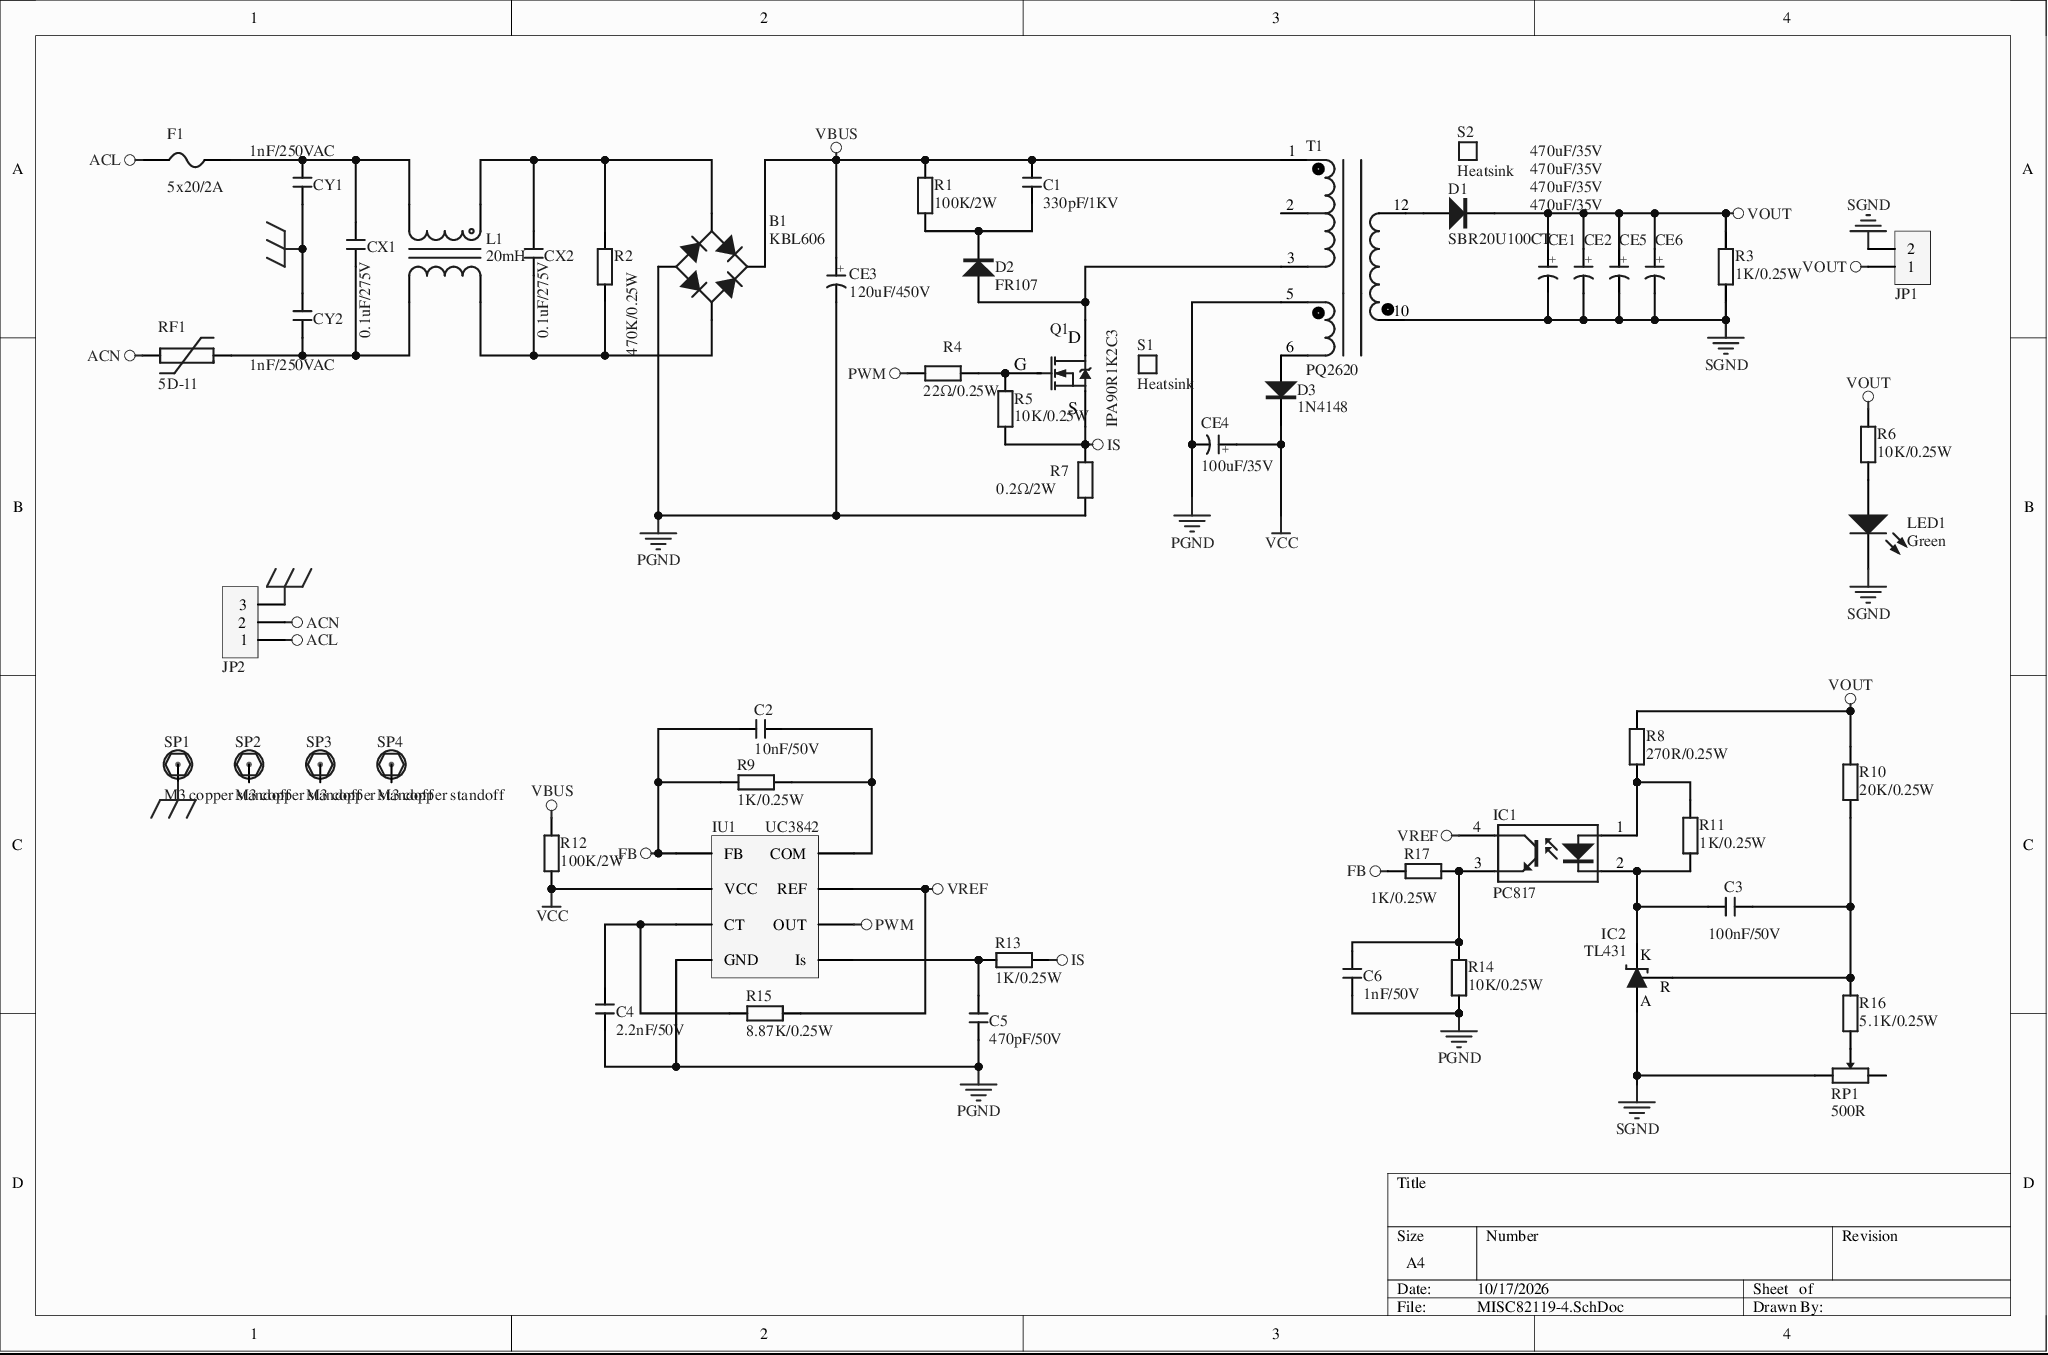
[diagram p0: MISC82119-4.SchDoc]
# Altium project MISC82119-10.PrjPcb
1 sheet, 55 parts. Net scope: global (net labels, ports and power ports of the same name join across sheets).
Board file: MISC82119.PcbDoc

## Sheet MISC82119-4.SchDoc
size A4

### Parts
B1  KBL606  [KBL]
C1  330pF/1KV  [CY 5*7*2.5]
C2  10nF/50V  [CC 2*5]
C3  100nF/50V  [CC 2*5]
C4  2.2nF/50V  [CC 2*5]
C5  470pF/50V  [CC 2*5]
C6  1nF/50V  [CC 2*5]
CE1  470uF/35V  [CAP 7.5*18*35.5]
CE2  470uF/35V  [CAP 7.5*18*35.5]
CE3  120uF/450V  [CAP 7.5*18*35.5]
CE4  100uF/35V  [CAP 7.5*18*35.5]
CE5  470uF/35V  [CAP 7.5*18*35.5]
CE6  470uF/35V  [CAP 7.5*18*35.5]
CX1  0.1uF/275V  [CX 10-13*11]
CX2  0.1uF/275V  [CX 10-13*11]
CY1  1nF/250VAC  [CY 7.5*8*4]
CY2  1nF/250VAC  [CY 7.5*8*4]
D1  SBR20U100CT  [TO220A]
D2  FR107  [DO-41]
D3  1N4148  [DO-35]
F1  5x20/2A  [FU 4x16_V]
IC1  PC817  [DIP4-300]
IC2  TL431  [TO92A]
IU1  UC3842  [DIP8-300]
JP1  HDR-1X2  [KF7620-2P]  (value not drawn)
JP2  HDR-1X3  [KF7620-3P]  (value not drawn)
L1  20mH  [UU10.5]
LED1  Green  [LED 3MM-G]
Q1  IPA90R1K2C3  [TO220A]
R1  100K/2W  [RS 2W-V6]
R2  470K/0.25W  [RS 1/4W]
R3  1K/0.25W  [RS 1/4W]
R4  22Ω/0.25W  [RS 1/4W]
R5  10K/0.25W  [RS 1/4W]
R6  10K/0.25W  [RS 1/4W]
R7  0.2Ω/2W  [RS 2W-V6]
R8  270R/0.25W  [RS 1/4W]
R9  1K/0.25W  [RS 1/4W]
R10  20K/0.25W  [RS 1/4W]
R11  1K/0.25W  [RS 1/4W]
R12  100K/2W  [RS 2W-V6]
R13  1K/0.25W  [RS 1/4W]
R14  10K/0.25W  [RS 1/4W]
R15  8.87K/0.25W  [RS 1/4W]
R16  5.1K/0.25W  [RS 1/4W]
R17  1K/0.25W  [RS 1/4W]
RF1  5D-11  [TVR-10D]
RP1  500R  [3296W]
S1  Heatsink  [SRP16-24-25-P]
S2  Heatsink  [SRP16-24-25-P]
SP1  M3 copper standoff  [M3x4+6_N]
SP2  M3 copper standoff  [M3x4+6_N]
SP3  M3 copper standoff  [M3x4+6_N]
SP4  M3 copper standoff  [M3x4+6_N]
T1  PQ2620  [PQ2625+6PIN]

### Nets
ACL: F1.2 JP2.1
ACN: JP2.2 RF1.1
FB: C2.1 IU1.2(FB) R9.2 R17.1
IS: Q1.3(S) R5.1 R7.2 R13.1
PE: CY1.1 CY2.2 JP2.3 SP1.1
PGND: B1.DC- C4.2 C5.2 C6.1 CE3.2(K) CE4.2(K) IU1.5(GND) R7.1 R14.2 T1.5
PWM: IU1.6(OUT) R4.2
SGND: CE1.2(K) CE2.2(K) CE5.2(K) CE6.2(K) IC2.2(A) JP1.2 LED1.2(K) R3.2 RP1.1 T1.10
VBUS: B1.DC+ C1.1 CE3.1(A) R1.2 R12.1 T1.1
VCC: CE4.1(A) D3.2(K) IU1.7(VCC) R12.2
VOUT: CE1.1(A) CE2.1(A) CE5.1(A) CE6.1(A) D1.2(K) JP1.1 R3.1 R6.2 R8.1 R10.1
VREF: IC1.4(C) IU1.8(REF) R15.2
NetB1_AC1: B1.AC1 CX2.2 L1.1 R2.1
NetB1_AC2: B1.AC2 CX2.1 L1.4 R2.2
NetC1_2: C1.2 D2.2(K) R1.1
NetC2_2: C2.2 IU1.1(COM) R9.1
NetC3_1: C3.1 IC1.2(K) IC2.3(K) R11.2
NetC3_2: C3.2 IC2.1(R) R10.2 R16.1
NetC4_1: C4.1 IU1.4(CT) R15.1
NetC5_1: C5.1 IU1.3(Is) R13.2
NetC6_2: C6.2 IC1.3(E) R14.1 R17.2
NetCX1_1: CX1.1 CY2.1 L1.3 RF1.2
NetCX1_2: CX1.2 CY1.2 F1.1 L1.2
NetD1_1: D1.1(A) T1.12
NetD2_1: D2.1(A) Q1.2(D) T1.3
NetD3_1: D3.1(A) T1.6
NetIC1_1: IC1.1(A) R8.2 R11.1
NetLED1_1: LED1.1(A) R6.1
NetQ1_1: Q1.1(G) R4.1 R5.2
NetR16_2: R16.2 RP1.2

Not connected (* = marked no-connect by the designer): RP1 3; SP2 1; SP3 1; SP4 1; T1 2

### Library data of the parts
B1 = KBL: 600V/8A bridge rectifier; BOM名称: 1KV/2A bridge rectifier
C1-C6 = CC: Ceramic disc capacitor; BOM名称: Through-hole ceramic disc capacitor
CE1-CE6 = CE: Through-hole electrolytic capacitor; BOM名称: Through-hole electrolytic capacitor
CX1 CX2 = CX: Safety X capacitor; BOM名称: X capacitor
CY1 CY2 = CY: Safety Y capacitor; BOM名称: High-voltage ceramic Y capacitor
D1-D3 = 1N4007: Rectifier diode; BOM名称: Rectifier diode
F1 = FU DIP: Through-hole fuse; BOM名称: Through-hole fuse
IC1 = 817: Linear optocoupler; BOM名称: Linear optocoupler
IC2 = TL431-ID: Adjustable precision shunt regulator; BOM名称: Adjustable precision shunt regulator
JP1 = Header 2: 2P connector; BOM名称: 2P connector
JP2 = Header 3: 3P connector; BOM名称: 3P connector
L1 = L-UU: Common-mode choke; BOM名称: Common-mode choke
LED1 = LED-3MM: Through-hole 3mm LED; BOM名称: Through-hole LED
Q1 = IRF840: N-channel MOSFET; BOM名称: N-channel MOSFET
R1-R17 = R-S: Color-band resistor; BOM名称: Color-band resistor
RF1 = PPTC: PPTC resettable fuse; BOM名称: PPTC resettable fuse
RP1 = RP: Single-gang potentiometer; BOM名称: Through-hole potentiometer
S1 S2 = S1: BOM名称: Heatsink
SP1-SP4 = 铜柱加头大焊盘: Copper standoff; BOM名称: Copper standoff
T1 = PQ2620: 12V high-frequency transformer; ROM名称: 12V high-frequency transformer